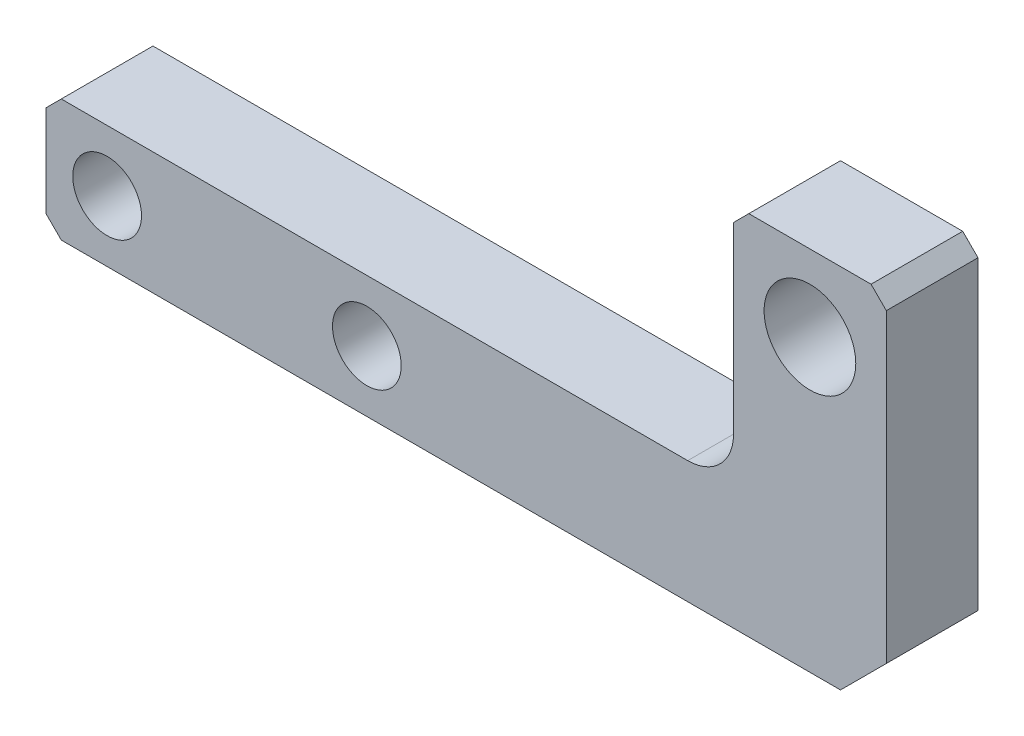
SolidWorks part; units mm, degrees
ref_plane "Front Plane" through (0, 0, 0) normal (0, 0, 1) x (1, 0, 0)
ref_plane "Top Plane" through (0, 0, 0) normal (0, 1, 0) x (1, 0, 0)
ref_plane "Right Plane" through (0, 0, 0) normal (1, 0, 0) x (0, 0, -1)
sketch "Sketch1" plane through (0, 0, 0) normal (0, 0, 1) x (1, 0, 0)
  line L0 (-55, 4) -> (-4.2226, 4) construction
  line L1 (0, 0) -> (-55, 0)
  line L2 (0, 0) -> (0, 24)
  line L3 (0, 24) -> (-10, 24)
  line L4 (-55, 0) -> (-55, 8)
  line L5 (-5, 24) -> (-5, 14) construction
  line L7 (-55, 8) -> (-10, 8)
  line L8 (-10, 24) -> (-10, 8)
  circle A0 centre (-51, 4) radius 2.25
  circle A1 centre (-34, 4) radius 2.25
  circle A2 centre (-5, 19) radius 3
  dimension "D5" = 4.5
  dimension "D9" = 6
  dimension "D1" = 8
  dimension "D2" = 55
  dimension "D3" = 10
  dimension "D4" = 24
  dimension "D6" = 4
  dimension "D7" = 17
  dimension "D8" = 19
extrude "Boss-Extrude1" add sketch "Sketch1" along normal mid plane 6
fillet "Fillet1" radius 3 1 edges at (-10, 8, 0)
chamfer "Chamfer1" distance 3 angle 45 1 edges at (0, 0, 0)
chamfer "Chamfer2" distance 1 angle 45 4 edges at (-55, 0, 0) (-55, 8, 0) (-10, 24, 0) (0, 24, 0)
